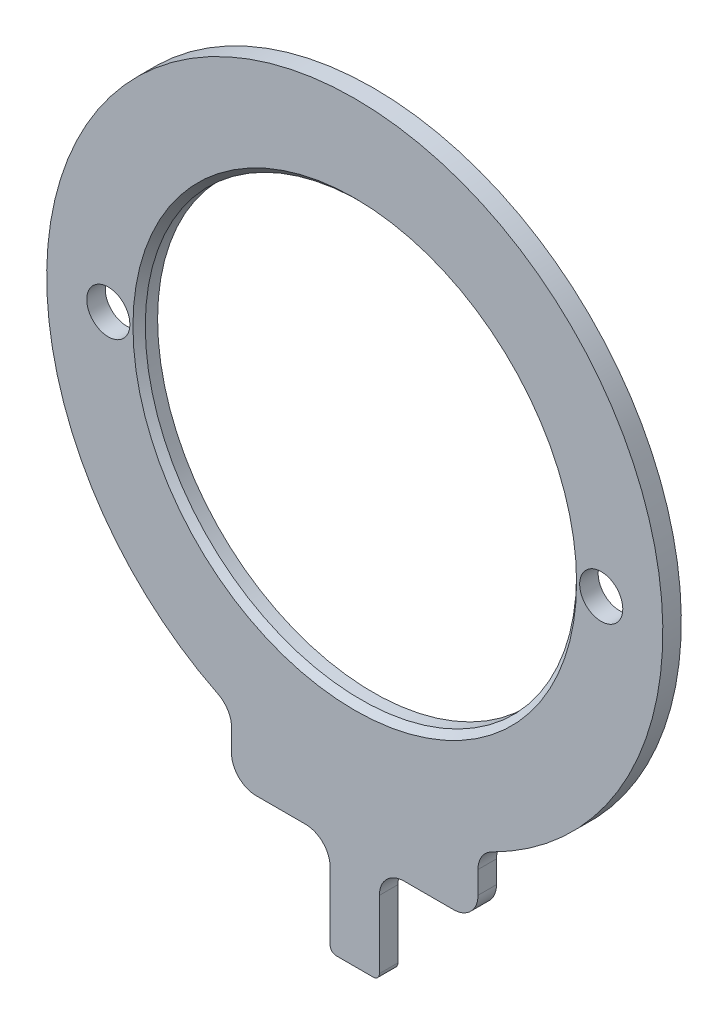
SolidWorks part; units mm, degrees
material "SUS 304"
ref_plane "前视基准面" through (0, 0, 0) normal (0, 0, 1) x (1, 0, 0)
ref_plane "上视基准面" through (0, 0, 0) normal (0, 1, 0) x (1, 0, 0)
ref_plane "右视基准面" through (0, 0, 0) normal (1, 0, 0) x (0, 0, -1)
sketch "草图1" plane through (0, 0, 0) normal (0, 0, 1) x (1, 0, 0)
  circle A0 centre (0, 0) radius 25
  circle A1 centre (0, 0) radius 17.5
  point P0 (0, 0)
  dimension "D1" = 50
  dimension "D2" = 35
extrude "凸台-拉伸1" add sketch "草图1" along normal blind 1.5
sketch "草图4" plane through (0, 0, 1.5) normal (0, 0, 1) x (1, 0, 0)
  line L1 (-10, -21) -> (10, -21)
  line L2 (-10, -21) -> (-10, -36)
  line L3 (-10, -36) -> (10, -36)
  line L4 (10, -21) -> (10, -36)
  dimension "D1" = 10
  dimension "D2" = 10
  dimension "D3" = 36
  dimension "D4" = 15
extrude "凸台-拉伸2" add sketch "草图4" against normal up to surface (1.5 mm away) up to face at (25, 0, 0)
sketch "草图5" plane through (0, 0, 1.5) normal (0, 0, 1) x (1, 0, 0)
  line L0 (10, -36) -> (10, -22.9129) construction
  line L1 (-10, -36) -> (-2, -36)
  line L2 (-10, -36) -> (-10, -28)
  line L3 (-10, -28) -> (-2, -28)
  line L4 (-2, -36) -> (-2, -28)
  line L5 (10, -36) -> (2, -36)
  line L6 (10, -36) -> (10, -28)
  line L7 (10, -28) -> (2, -28)
  line L8 (2, -36) -> (2, -28)
  line L9 (-10, -36) -> (10, -36) construction
  dimension "D1" = 8
  dimension "D2" = 8
  dimension "D4" = 8
extrude "切除-拉伸3" cut sketch "草图5" against normal blind 20
fillet "圆角2" radius 2 6 edges at (-2, -28, 0.75) (2, -28, 0.75) (-10, -28, 0.75) (-10, -22.9129, 0.75) (10, -28, 0.75) (10, -22.9129, 0.75)
sketch "草图6" plane through (0, 0, 1.5) normal (0, 0, 1) x (1, 0, 0)
  circle A0 centre (-20, 0) radius 1.75
  circle A1 centre (20, 0) radius 1.75
  dimension "D1" = 3.5
  dimension "D2" = 3.5
  dimension "D4" = 20
  dimension "D3" = 20
extrude "切除-拉伸4" cut sketch "草图6" against normal blind 40
fillet "圆角3" radius 0.5 2 edges at (2, -36, 0.75) (-2, -36, 0.75)
chamfer "倒角1" distance 0.5 angle 45 1 edges at (17.5, 0, 1.5)
